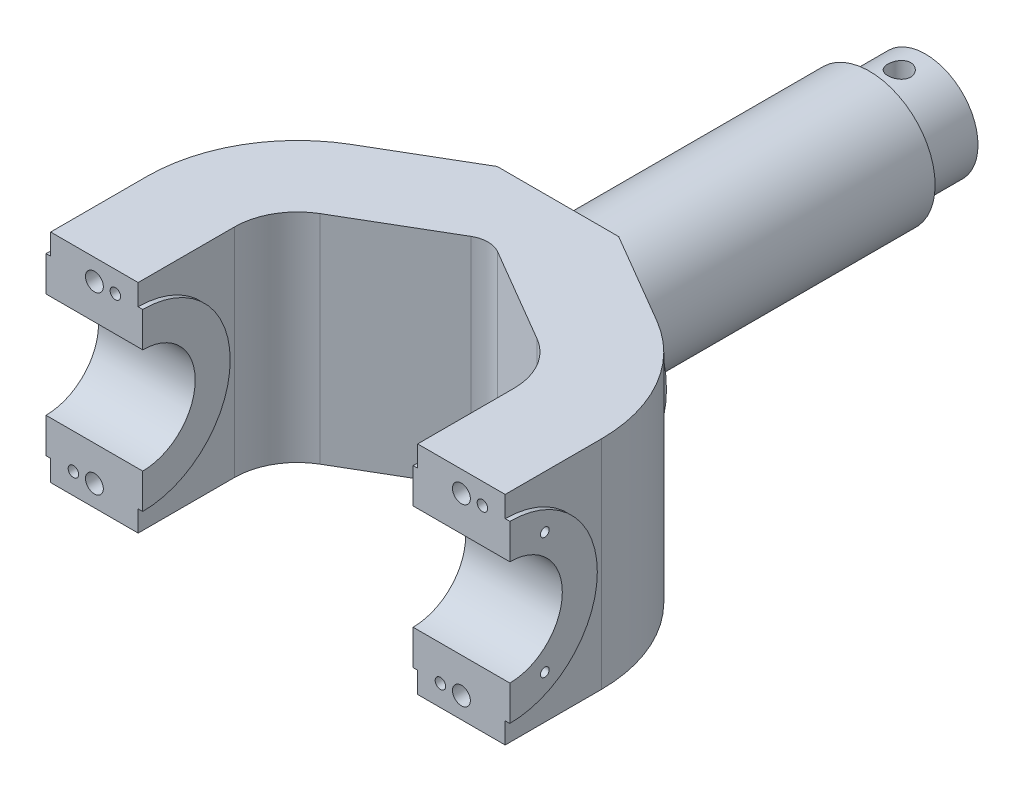
from build123d import *

# Parameters (mm, degrees)
BOSS_EXTRUDE1_DEPTH         = 62
SKETCH2_R                   = 62
BOSS_EXTRUDE2_DEPTH         = 15.974431
SKETCH3_R                   = 37.5
BOSS_EXTRUDE3_DEPTH         = 178
SKETCH4_R                   = 30
BOSS_EXTRUDE4_DEPTH         = 210
CUT_EXTRUDE1_DEPTH          = 255.568306158
CUT_EXTRUDE1_DEPTH_BACK     = 255.568306158
SKETCH5_R                   = 6.5
BOSS_EXTRUDE5_DEPTH         = 132.5
CUT_EXTRUDE2_DEPTH          = 77.25
CUT_EXTRUDE3_DEPTH          = 256.930166338
CUT_EXTRUDE3_DEPTH_BACK     = 256.930166338
M6_TAPPED_HOLE1_AT_2_COUNT  = 2
M6_TAPPED_HOLE1_AT_2_PITCH  = 69.282032303
M12_TAPPED_HOLE1_D          = 10.2
M12_TAPPED_HOLE1_DEPTH      = 36.75
M12_TAPPED_HOLE1_TIP        = 3.064389157
F_6MM_BLIND_PIN_HOLE1_D     = 6
F_6MM_BLIND_PIN_HOLE1_DEPTH = 15
F_6MM_BLIND_PIN_HOLE1_TIP   = 1.802581857
CHAMFER1_SIZE               = 2
FILLET1_R                   = 3


with BuildPart() as part:
    # Sketch1 → Boss-Extrude1 (new, symmetric)
    with BuildSketch(Plane(origin=(0, 0, 0), x_dir=(1, 0, 0), z_dir=(0, 1, 0))):
        with BuildLine():
            Line((-129.85, -160), (-79.85, -160))
            Line((-79.85, -160), (-79.85, -105))
            ThreePointArc((-79.85, -105), (-75.080495551, -87.093125688), (-62.035769577, -73.931080081))
            Line((-62.035769577, -73.931080081), (-7.57740399, -42.054616701))
            ThreePointArc((-7.57740399, -42.054616701), (0, -40), (7.57740399, -42.054616701))
            Line((7.57740399, -42.054616701), (62.035769577, -73.931080081))
            ThreePointArc((62.035769577, -73.931080081), (75.080495551, -87.093125688), (79.85, -105))
            Line((79.85, -105), (79.85, -160))
            Line((79.85, -160), (129.85, -160))
            Line((129.85, -160), (129.85, -105))
            ThreePointArc((129.85, -105), (118.456183817, -62.222466922), (87.293782877, -30.779802417))
            Line((87.293782877, -30.779802417), (34.708974059, 0))
            Line((34.708974059, 0), (-34.708974059, 0))
            Line((-34.708974059, 0), (-87.293782877, -30.779802417))
            ThreePointArc((-87.293782877, -30.779802417), (-118.456183817, -62.222466922), (-129.85, -105))
            Line((-129.85, -105), (-129.85, -160))
        make_face()
    extrude(amount=BOSS_EXTRUDE1_DEPTH, both=True)

    # Sketch2 → Boss-Extrude2 (add)
    with BuildSketch(Plane.XY):
        Circle(SKETCH2_R)
    extrude(amount=BOSS_EXTRUDE2_DEPTH)

    # Sketch3 → Boss-Extrude3 (add)
    with BuildSketch(Plane.XY):
        Circle(SKETCH3_R)
    extrude(amount=-BOSS_EXTRUDE3_DEPTH)

    # Sketch4 → Boss-Extrude4 (add)
    with BuildSketch(Plane.XY):
        Circle(SKETCH4_R)
    extrude(amount=-BOSS_EXTRUDE4_DEPTH)

    # Sketch5 → Cut-Extrude1 (cut, two sides: drawn at the far end of the back side and taken through both)
    with BuildSketch(Plane(origin=(0, 0, 0), x_dir=(1, 0, 0), z_dir=(0, 1, 0)).offset(-CUT_EXTRUDE1_DEPTH_BACK)):
        with Locations(Location((0, 195, 0), (0, 0, 270))):
            Circle(SKETCH5_R)
    extrude(amount=CUT_EXTRUDE1_DEPTH + CUT_EXTRUDE1_DEPTH_BACK, mode=Mode.SUBTRACT)

    # Sketch6 → Boss-Extrude5 (add, symmetric)
    with BuildSketch(Plane(origin=(0, 0, 0), x_dir=(0, 0, -1), z_dir=(1, 0, 0))):
        with BuildLine():
            Line((-160, 50), (-160, 30))
            ThreePointArc((-160, 30), (-130, 0), (-160, -30))
            Line((-160, -30), (-160, -50))
            ThreePointArc((-160, -50), (-110, 0), (-160, 50))
        make_face()
    extrude(amount=BOSS_EXTRUDE5_DEPTH, both=True)

    # Sketch7 → Cut-Extrude2 (cut, symmetric)
    with BuildSketch(Plane(origin=(0, 0, 0), x_dir=(0, 0, -1), z_dir=(1, 0, 0))):
        with BuildLine():
            Line((-160, 28), (-160, 52))
            ThreePointArc((-160, 52), (-108, 0), (-160, -52))
            Line((-160, -52), (-160, -28))
            ThreePointArc((-160, -28), (-132, 0), (-160, 28))
        make_face()
    extrude(amount=CUT_EXTRUDE2_DEPTH, both=True, mode=Mode.SUBTRACT)

    # Sketch15 → Cut-Extrude3 (cut, two sides: drawn at the far end of the back side and taken through both)
    with BuildSketch(Plane(origin=(0, 0, 0), x_dir=(0, 0, -1), z_dir=(1, 0, 0)).offset(-CUT_EXTRUDE3_DEPTH_BACK)):
        with BuildLine():
            Line((-160, 30), (-160, -30))
            ThreePointArc((-160, -30), (-130, 0), (-160, 30))
        make_face()
    extrude(amount=CUT_EXTRUDE3_DEPTH + CUT_EXTRUDE3_DEPTH_BACK, mode=Mode.SUBTRACT)

    # Sketch8 → M6 Tapped Hole1 (revolve, cut)
    with BuildSketch(Plane(origin=(132.5, 34.641016151, 140), x_dir=(0, 0, -1), z_dir=(0, 1, 0))):
        Polygon((0, 0), (0, 18.502151548), (2.5, 17), (2.5, 0), align=None)
    m6_tapped_hole1 = revolve(axis=Axis((138.85, 34.641016151, 140), (-1, 0, 0)), mode=Mode.SUBTRACT)

    # M6 Tapped Hole1 at 2: M6 Tapped Hole1 ×2
    with Locations(*[(0, -i * M6_TAPPED_HOLE1_AT_2_PITCH, 0) for i in range(1, M6_TAPPED_HOLE1_AT_2_COUNT)]):
        add(m6_tapped_hole1, mode=Mode.SUBTRACT)

    # Mirror1: M6 Tapped Hole1 across plane
    add(m6_tapped_hole1.mirror(Plane(origin=(0, 0, 0), x_dir=(0, 0, 1), z_dir=(1, 0, 0))), mode=Mode.SUBTRACT)

    # Mirror1 copy 1 sketch → Mirror1 copy 1 (revolve, cut)
    with BuildSketch(Plane(origin=(-132.5, -34.641016151, 140), x_dir=(0, 0, -1), z_dir=(0, 1, 0))):
        Polygon((0, 0), (0, -18.502151548), (2.5, -17), (2.5, 0), align=None)
    revolve(axis=Axis((-138.85, -34.641016151, 140), (-1, 0, 0)), mode=Mode.SUBTRACT)

    # M12 Tapped Hole1
    with Locations(Plane.XY.offset(160)):
        with Locations((104.85, 50), (104.85, -50), (-104.85, 50), (-104.85, -50)):
            Hole(M12_TAPPED_HOLE1_D / 2, depth=M12_TAPPED_HOLE1_DEPTH)
            with Locations((0, 0, -(M12_TAPPED_HOLE1_DEPTH + M12_TAPPED_HOLE1_TIP / 2))):  # 118° drill point
                Cone(0, M12_TAPPED_HOLE1_D / 2, M12_TAPPED_HOLE1_TIP, mode=Mode.SUBTRACT)

    # 6mm blind pin hole1
    with Locations(Plane.XY.offset(160)):
        with Locations((116.85, 50), (92.85, -50), (-92.85, 50), (-116.85, -50)):
            Hole(F_6MM_BLIND_PIN_HOLE1_D / 2, depth=F_6MM_BLIND_PIN_HOLE1_DEPTH)
            with Locations((0, 0, -(F_6MM_BLIND_PIN_HOLE1_DEPTH + F_6MM_BLIND_PIN_HOLE1_TIP / 2))):  # 118° drill point
                Cone(0, F_6MM_BLIND_PIN_HOLE1_D / 2, F_6MM_BLIND_PIN_HOLE1_TIP, mode=Mode.SUBTRACT)

    # Chamfer1
    chamfer1_edges = [part.edges().sort_by_distance(p)[0] for p in [
        (-30, 0, -178),
    ]]
    chamfer(chamfer1_edges, length=CHAMFER1_SIZE)

    # Fillet1
    fillet1_edges = [part.edges().sort_by_distance(p)[0] for p in [
        (-37.5, 0, 0),
    ]]
    fillet(fillet1_edges, radius=FILLET1_R)


solid = part.part
